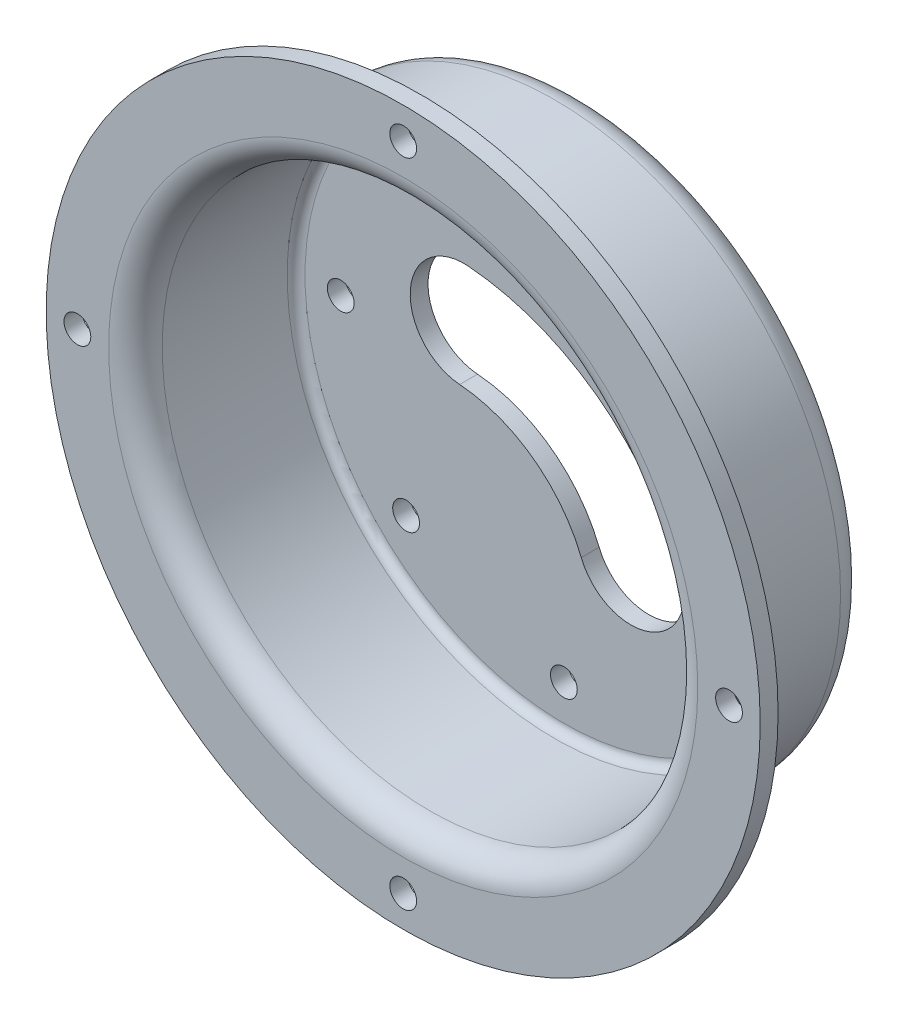
from build123d import *

# Parameters (mm, degrees)
SKETCH1_R           = 160
SKETCH1_R_2         = 7.5
BOSS_EXTRUDE1_DEPTH = 10
SKETCH2_R           = 160
SKETCH2_R_2         = 150
BOSS_EXTRUDE2_DEPTH = 80
SKETCH3_R           = 200
SKETCH3_R_2         = 150
SKETCH3_R_3         = 7.5
BOSS_EXTRUDE3_DEPTH = 10
FILLET1_R           = 5
FILLET2_R           = 15


with BuildPart() as part:
    # Sketch1 → Boss-Extrude1 (new body)
    with BuildSketch(Plane.XY):
        Circle(SKETCH1_R)
        with Locations((0, 125)):
            Circle(SKETCH1_R_2, mode=Mode.SUBTRACT)
        with Locations((88.388347648, 88.388347648)):
            Circle(SKETCH1_R_2, mode=Mode.SUBTRACT)
        with Locations((125, 0)):
            Circle(SKETCH1_R_2, mode=Mode.SUBTRACT)
        with Locations((88.388347648, -88.388347648)):
            Circle(SKETCH1_R_2, mode=Mode.SUBTRACT)
        with Locations((0, -125)):
            Circle(SKETCH1_R_2, mode=Mode.SUBTRACT)
        with Locations((-88.388347648, -88.388347648)):
            Circle(SKETCH1_R_2, mode=Mode.SUBTRACT)
        with Locations((-125, 0)):
            Circle(SKETCH1_R_2, mode=Mode.SUBTRACT)
        with Locations((-88.388347648, 88.388347648)):
            Circle(SKETCH1_R_2, mode=Mode.SUBTRACT)
        with BuildLine():
            ThreePointArc((-53.803098946, 50.037724546), (-86.000050805, 22.408821364), (-58.371147623, -9.788130495))
            ThreePointArc((-58.371147623, -9.788130495), (-17.190203431, -25.016114851), (9.751908775, -59.684317313))
            ThreePointArc((9.751908775, -59.684317313), (48.783936726, -76.312630338), (65.412249751, -37.280602387))
            ThreePointArc((65.412249751, -37.280602387), (18.26355339, 23.388751922), (-53.803098946, 50.037724546))
        make_face(mode=Mode.SUBTRACT)
    extrude(amount=BOSS_EXTRUDE1_DEPTH)

    # Sketch2 → Boss-Extrude2 (add)
    with BuildSketch(Plane.XY.offset(10)):
        Circle(SKETCH2_R)
        Circle(SKETCH2_R_2, mode=Mode.SUBTRACT)
    extrude(amount=BOSS_EXTRUDE2_DEPTH)

    # Sketch3 → Boss-Extrude3 (add)
    with BuildSketch(Plane.XY.offset(90)):
        Circle(SKETCH3_R)
        Circle(SKETCH3_R_2, mode=Mode.SUBTRACT)
        with Locations((0, 182.5)):
            Circle(SKETCH3_R_3, mode=Mode.SUBTRACT)
        with Locations((182.5, 0)):
            Circle(SKETCH3_R_3, mode=Mode.SUBTRACT)
        with Locations((0, -182.5)):
            Circle(SKETCH3_R_3, mode=Mode.SUBTRACT)
        with Locations((-182.5, 0)):
            Circle(SKETCH3_R_3, mode=Mode.SUBTRACT)
    extrude(amount=BOSS_EXTRUDE3_DEPTH)

    # Fillet1
    fillet1_edges = [part.edges().sort_by_distance(p)[0] for p in [
        (-150, 0, 10),
        (-160, 0, 90),
    ]]
    fillet(fillet1_edges, radius=FILLET1_R)

    # Fillet2
    fillet2_edges = [part.edges().sort_by_distance(p)[0] for p in [
        (-160, 0, 0),
        (-150, 0, 100),
    ]]
    fillet(fillet2_edges, radius=FILLET2_R)


solid = part.part
